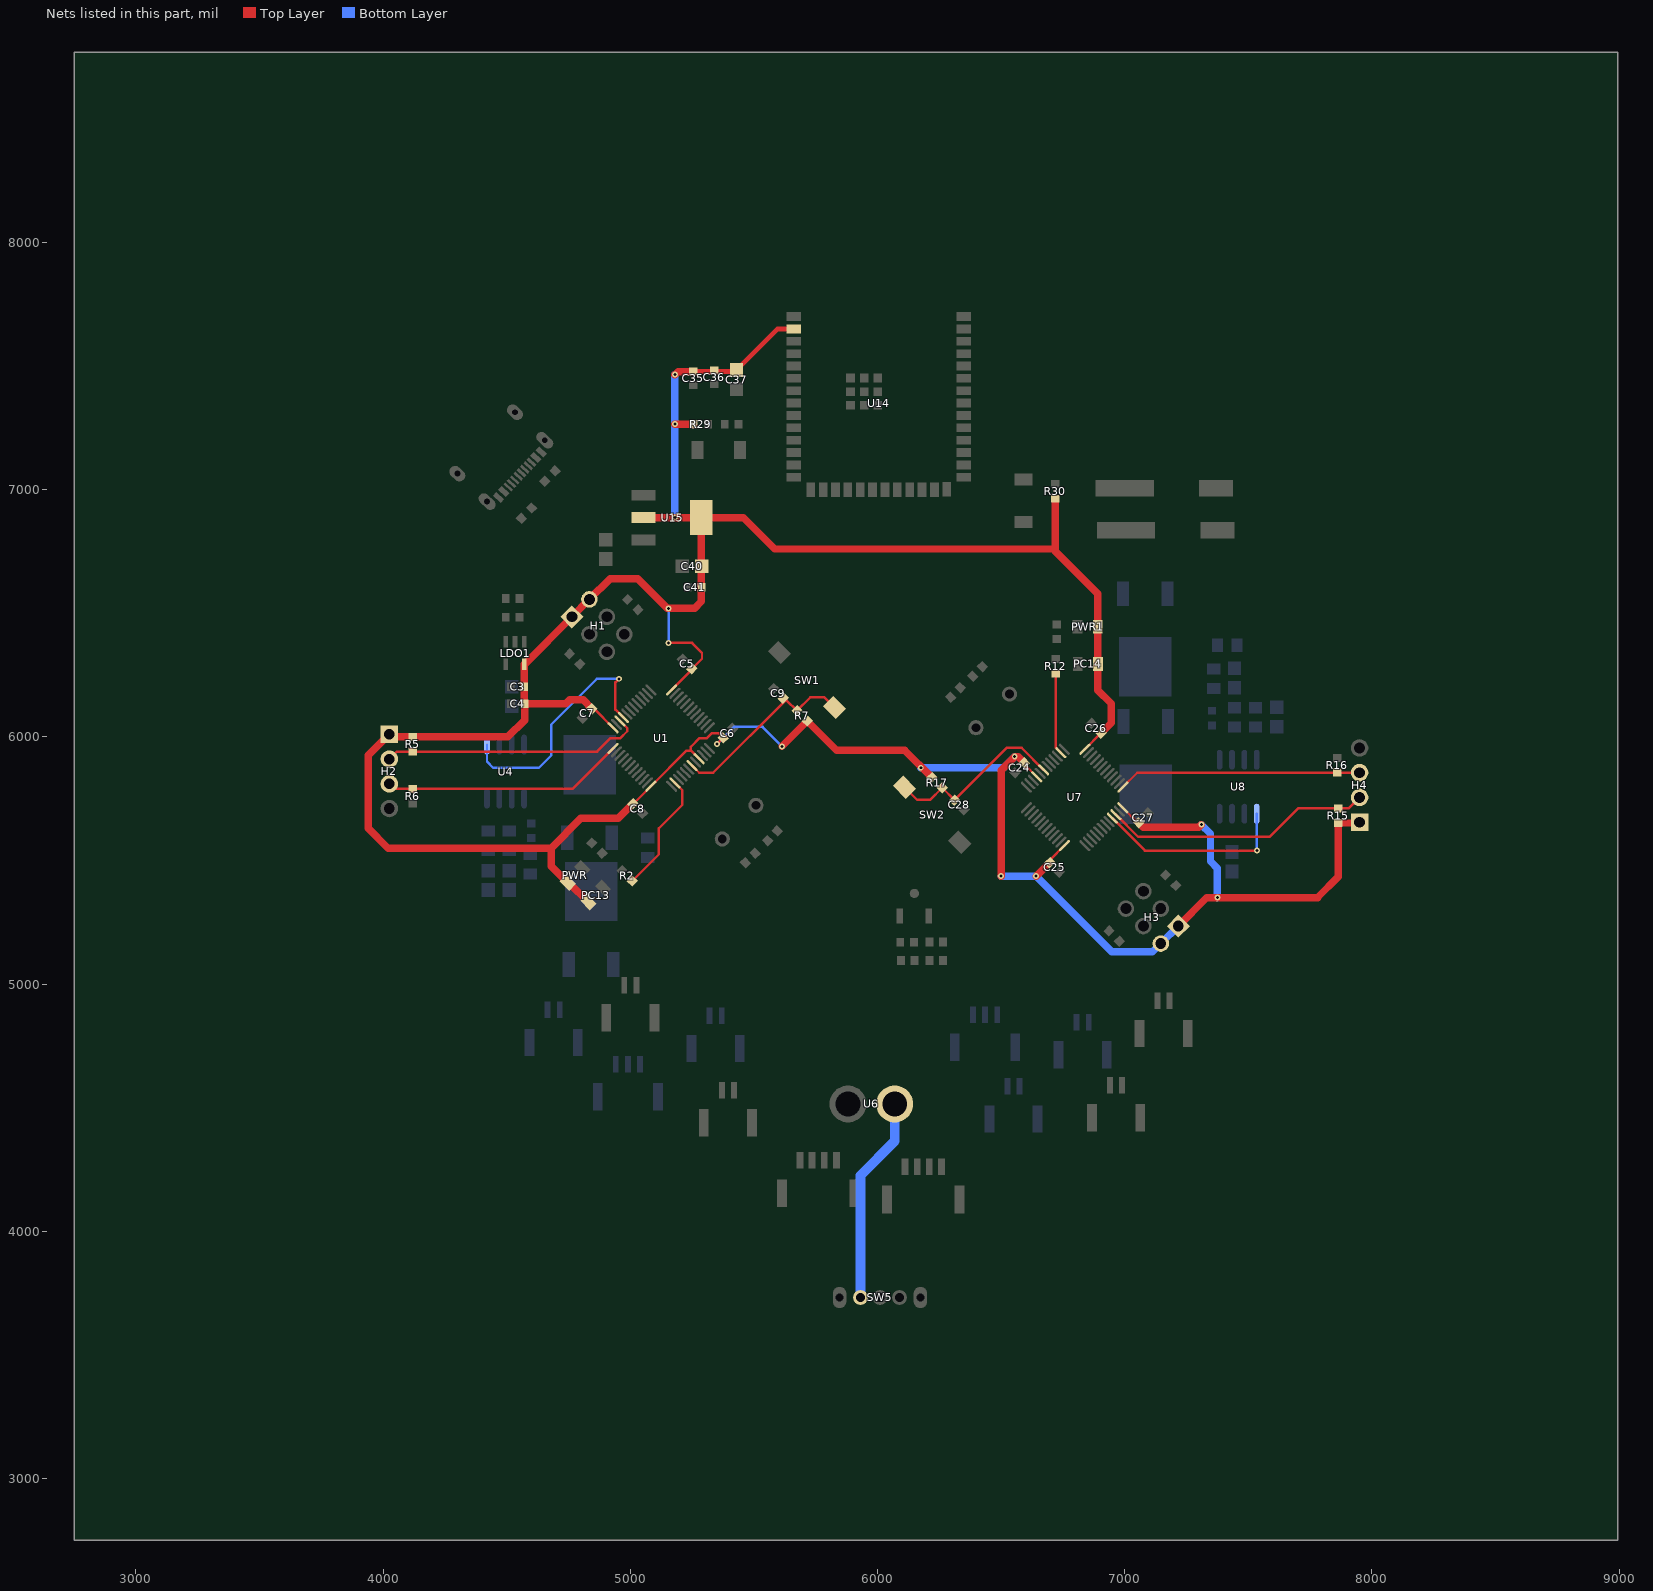
[diagram p0: the nets of this part, all layers, seen from the top]
# Altium PCB MISC62500.pcbdoc (part 3 of 3)
Units mil, origin at the board's own origin, x right, y up, seen from the top; angles counter-clockwise.
Board outline 6245 x 6020 mil, 2 copper layers (Top Layer, Bottom Layer), stack 62.206 mil thick; 106 components, 73 nets, 432 pads, 293 vias.

## Via types
v1: diameter 24, hole 12, Top Layer to Bottom Layer, 293 vias

## Nets (pads, with @x,y where several pads share a name; then routed paths per layer and width w, separated by ;. In a path a pad name is that pad's centre, name@x,y a point inside that pad or via, vN(x,y) a via of type N, cw(c..) or ccw(c..) an arc to the next point about the centre after c; other vN are vias at no path point) (continued)
PA12: U1.33 U4.1 | length 1012.2
  Top Layer w10: v1(4955,6235) 4940,6220 4940,6110.41 U1.33@4971.89,6078.52
  Bottom Layer w10: U4.1@4420.26,5968.7 4420.26,5899.74 4445,5875 4630,5875 4680,5925 4680,6050 4865,6235 v1(4955,6235)
PA12B: U7.33 U8.1 | length 788.7
  Top Layer w10: U7.33@6950.41,5671.45 7081.86,5540 v1(7535,5540)
  Bottom Layer w10: U8.1@7533.98,5689.22 7535,5688.19 v1(7535,5540)
PC13: R2.2 U1.2 | length 492.8
  Top Layer w10: R2.2@5007.92,5417.08 5115,5524.16 5115,5630 5210,5725 5210,5784.73 U1.2@5180.68,5814.05
PC13B: R12.2 U7.2 | length 328
  Top Layer w10: R12.2@6720.9,6255.3 6720.9,5956.63 U7.2@6741.62,5935.91
POWER: SW5.1 U6.2 | length 840
  Bottom Layer w40: SW5.1@5931.26,3732.22 5931.26,4226.26 6069.48,4364.48 U6.2@6069.48,4515
RESET: C9.2 R7.1 SW1.1 U1.7 | length 765.8
  Top Layer w10: U1.7@5250.27,5883.64 5278.92,5855 5335,5855 5627.5,6147.5 5632.5,6147.5 R7.1@5674.03,6105.97 5728.05,6160 5785,6160 SW1.1@5826.36,6118.64
RESETB: C28.2 R17.1 SW2.1 U7.7 | length 748.5
  Top Layer w10: SW2.1@6109.55,5796.32 6160.87,5745 6212.89,5745 R17.1@6261.88,5793.99 C28.2@6311.42,5744.45 6521.97,5955 6583.35,5955 U7.7@6672.03,5866.32
SWCLK: H2.3 R6.2 U1.37 | length 981.4
  Top Layer w10: H2.3@4025,5810 4045.46,5789.54 R6.2@4120.5,5789.54 4766.42,5789.54 U1.37@4930.13,5953.25
SWCLKB: H4.3 R16.2 U7.37 | length 982
  Top Layer w10: U7.37@6992.17,5796.72 7050.46,5855 H4.3@7950,5855
SWIO: H2.2 R5.1 U1.34 | length 1063.4
  Top Layer w10: H2.2@4025,5910 4055.34,5940.34 R5.1@4120,5940.34 4865.34,5940.34 4920,5995 4960,5995 4987.5,6022.5 4987.5,6035.06 U1.34@4957.97,6064.59
SWIOB: H4.2 R15.1 U7.34 | length 1089.4
  Top Layer w10: U7.34@6964.34,5685.37 7054.7,5595 7585,5595 7700.9,5710.9 R15.1@7864.5,5710.9 7905.9,5710.9 H4.2@7950,5755
VCC: C3.2 C4.2 C5.2 C6.2 C7.2 C8.2 C24.2 C25.2 C26.2 C27.2 C35.2 C36.2 C37.2 C40.2 C41.1 H1.1 H1.2 H2.1 H3.1 H3.2 H4.1 LDO1.5 PC13.1 PC14.1 PWR1.1 PWR.1 R5.2 R7.2 R15.2 R17.2 R29.1 R30.1 U1.9 U1.24 U1.36 U1.48 U7.9 U7.24 U7.36 U7.48 U14.2 U15.2 U15.4 | length 14369.7
  Top Layer w10: C7.2@4844.49,6114.49 4852.4,6114.49 U1.36@4930.13,6036.75 ; C8.2@5012.6,5729.49 U1.48@5083.25,5800.13 5227.71,5944.59 5245,5944.59 ; v1(5155,6380) 5250,6380 5290,6340 5290,6316.02 C5.2@5249.49,6275.51 5249.49,6272.6 U1.24@5166.75,6189.87 ; U1.9@5278.11,5911.48 5245,5944.59 ; v1(5350.87,5970.87) C6.2@5375.51,5995.51 5356.02,6015 5330,6015 5310,5995 5280,5995 5245,5960 5245,5944.59 ; C24.2@6594.49,5888.18 U7.9@6644.19,5838.48 ; C25.2@6697.03,5491.68 6697.03,5501.58 U7.24@6755.55,5560.09 ; U7.48@6839.06,5949.83 6904.49,6015.26 C26.2@6904.49,6015.51 ; U7.36@6992.17,5713.21 7052.3,5653.08 C27.2@7056.01,5653.08
  Top Layer w20: C35.2@5255,7477.56 5423.19,7477.56 C37.2@5430,7484.37 5595.82,7650.19 U14.2@5660.51,7650.19
  Top Layer w30: PC13.1@4830.76,5330.76 4751.11,5410.42 PWR.1@4746.57,5410.42 4680,5476.99 4680,5550 ; C7.2@4844.49,6114.49 4808.98,6150 4755,6150 4738.68,6133.68 C4.2@4572.53,6133.68 ; C8.2@5010.51,5729.49 4951.02,5670 4800,5670 4680,5550 ; U15.2@5053.04,6887.1 v1(5180.55,6887.1) U15.4@5286.89,6887.1 ; v1(5180,7265) R29.1@5255.34,7265 ; v1(5180.55,7465) 5193.11,7477.56 C35.2@5255,7477.56 ; v1(5613.65,5961.71) R7.2@5715.97,6064.03 5835,5945 6110.87,5945 R17.2@6219.93,5835.93 ; v1(6500,5436.38) 6500,5865 v1(6555,5920) 6568.98,5920 C24.2@6594.49,5894.49 ; v1(6641.73,5436.38) C25.2@6697.03,5491.68 ; R30.1@6719.59,6963.01 6719.59,6760 ; C26.2@6904.49,6015.51 6945,6056.02 6945,6135 6891.35,6188.65 PWR1.1@6891.35,6445 6891.35,6578.65 6719.59,6750.41 6719.59,6760 ; C27.2@7056.01,5653.08 7074.09,5635 7300,5635 v1(7310,5645) ; H3.1@7216.97,5234.61 7332.36,5350 v1(7375,5350) 7780,5350 7864.5,5434.5 R15.2@7864.5,5651.58 7946.58,5651.58 H4.1@7950,5655 ; C4.2@4572.53,6133.68 4571.08,6135.13 LDO1.5@4571.08,6293.81 4572.39,6293.81 H1.1@4763.93,6485.36 H1.2@4834.64,6556.07 4918.58,6640 5030,6640 5150,6520 5260,6520 5287.56,6547.56 C41.1@5287.56,6605 5287.56,6886.44 U15.4@5286.89,6887.1 ; C4.2@4572.53,6133.68 4572.53,6067.53 4504.66,5999.66 R5.2@4120,5999.66 4035.34,5999.66 H2.1@4025,6010 3940,5925 3940,5630 4020,5550 4680,5550 ; U15.4@5286.89,6887.1 5457.9,6887.1 5585,6760 6719.59,6760
  Bottom Layer w10: v1(5155,6380) v1(5155,6520) ; v1(5350.87,5970.87) 5420,6040 5535.36,6040 v1(5613.65,5961.71)
  Bottom Layer w30: v1(5180.55,6887.1) v1(5180.55,7465) ; v1(6175,5875) 6510,5875 v1(6555,5920) ; v1(6500,5436.38) v1(6641.73,5436.38) 6948.12,5130 7112.36,5130 H3.2@7146.26,5163.9 H3.1@7216.97,5234.61 ; v1(7310,5645) 7347,5608 7347,5496.33 7375,5468.33 v1(7375,5350)
pads on no net: LDO1.4 SW5.3 U1.3 U1.4 U1.10 U1.11 U1.14 U1.15 U1.17 U1.18 U1.19 U1.25 U1.26 U1.27 U1.28 U1.38 U1.39 U1.40 U1.41 U1.42 U1.43 U1.45 U1.46 U7.3 U7.4 U7.10 U7.11 U7.14 U7.15 U7.17 U7.18 U7.19 U7.25 U7.26 U7.27 U7.28 U7.38 U7.39 U7.40 U7.41 U7.42 U7.43 U7.45 U7.46 U14.6 U14.7 U14.15 U14.16 U14.18 U14.19 U14.20 U14.21 U14.22 U14.23 U14.24 U14.25 U14.26 U14.28 U14.29 U14.30 U14.31 U14.32 U14.33 U14.34 U14.35 U14.36 U14.37 U14.38 U14.39 USB1.A8 USB1.B8

## Polygon pours and split planes (outlines as drawn)
GND on Top Layer (solid, remove dead copper, pour order 0): 3000,8520 3000,3000 8745,3000 8745,8520
GND on Bottom Layer (solid, remove dead copper, pour order 2): 3545,8185 3545,3300 8260,3300 8260,8185

## Keep-outs
Board Outline Layer:
  drawing of 90 lines, arcs and shapes, not listed

## Silkscreen, mask and mechanical layers (free items; w line width, h text height)
Mechanical Layer:
  circle w0.1: c5530.51,5039.63 r61.02
  circle w0.1: c6475.41,6614.41 r61.02
  circle w0.1: c4743.1,4366.1 r49.21
  circle w0.1: c7124.98,4257.75 r49.21
  circle w0.1: c4880.94,7396.29 r49.21
  circle w0.1: c7262.82,7287.94 r49.21
  circle w0.1: c4118.1,6394.72 r62.99
  circle w0.1: c5435.26,3942.16 r62.99
  circle w0.1: c7887.83,5259.32 r62.99
  circle w0.1: c7125.03,7396.26 r49.21
  circle w0.1: c4268.77,6758.45 r62.99
  circle w0.1: c5071.53,4092.82 r62.99
  circle w0.1: c7737.16,4895.59 r62.99
  circle w0.1: c6570.66,7711.88 r62.99
  circle w0.1: c6934.39,7561.22 r62.99
  circle w0.1: c7887.84,6394.66 r62.99
  circle w0.1: c6570.6,3942.14 r62.99
  circle w0.1: c4118.08,5259.38 r62.99
  circle w0.1: c5435.32,7711.9 r62.99
  circle w0.1: c7737.18,6758.4 r62.99
  circle w0.1: c6934.34,4092.8 r62.99
  circle w0.1: c4268.74,4895.64 r62.99
  circle w0.1: c5071.58,7561.24 r62.99
  circle w0.1: c4743.14,7287.98 r49.21
  circle w0.1: c7262.78,4366.06 r49.21
  circle w0.1: c4880.89,4257.78 r49.21
  circle w0.1: c5530.53,6614.43 r61.02
  circle w0.1: c6475.39,5039.61 r61.02